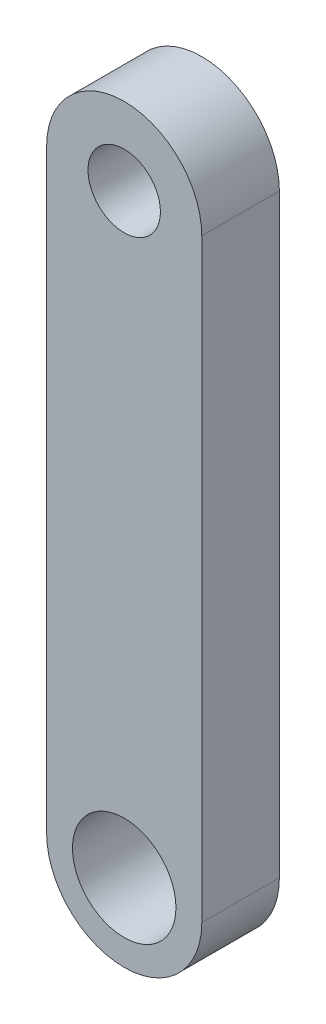
SolidWorks part; units mm, degrees
ref_plane "前视基准面" through (0, 0, 0) normal (0, 0, 1) x (1, 0, 0)
ref_plane "上视基准面" through (0, 0, 0) normal (0, 1, 0) x (1, 0, 0)
ref_plane "右视基准面" through (0, 0, 0) normal (1, 0, 0) x (0, 0, -1)
sketch "草图1" plane through (0, 0, 0) normal (0, 0, 1) x (1, 0, 0)
  line L0 (0, 0) -> (0, 115) construction
  line L1 (-15, 0) -> (-15, 115)
  line L2 (15, 0) -> (15, 115)
  arc A0 (-15, 0) -> (15, 0) centre (0, 0) ccw
  arc A1 (15, 115) -> (-15, 115) centre (0, 115) ccw
  point P3 (0, 57.5)
  dimension "D2" = 15
  dimension "D1" = 115
extrude "凸台-拉伸1" add sketch "草图1" along normal blind 15
sketch "草图2" plane through (0, 0, 15) normal (0, 0, 1) x (1, 0, 0)
  circle A0 centre (0, 115) radius 7
  circle A1 centre (0, 0) radius 10
  dimension "D1" = 14
  dimension "D2" = 20
extrude "切除-拉伸1" cut sketch "草图2" against normal through all
